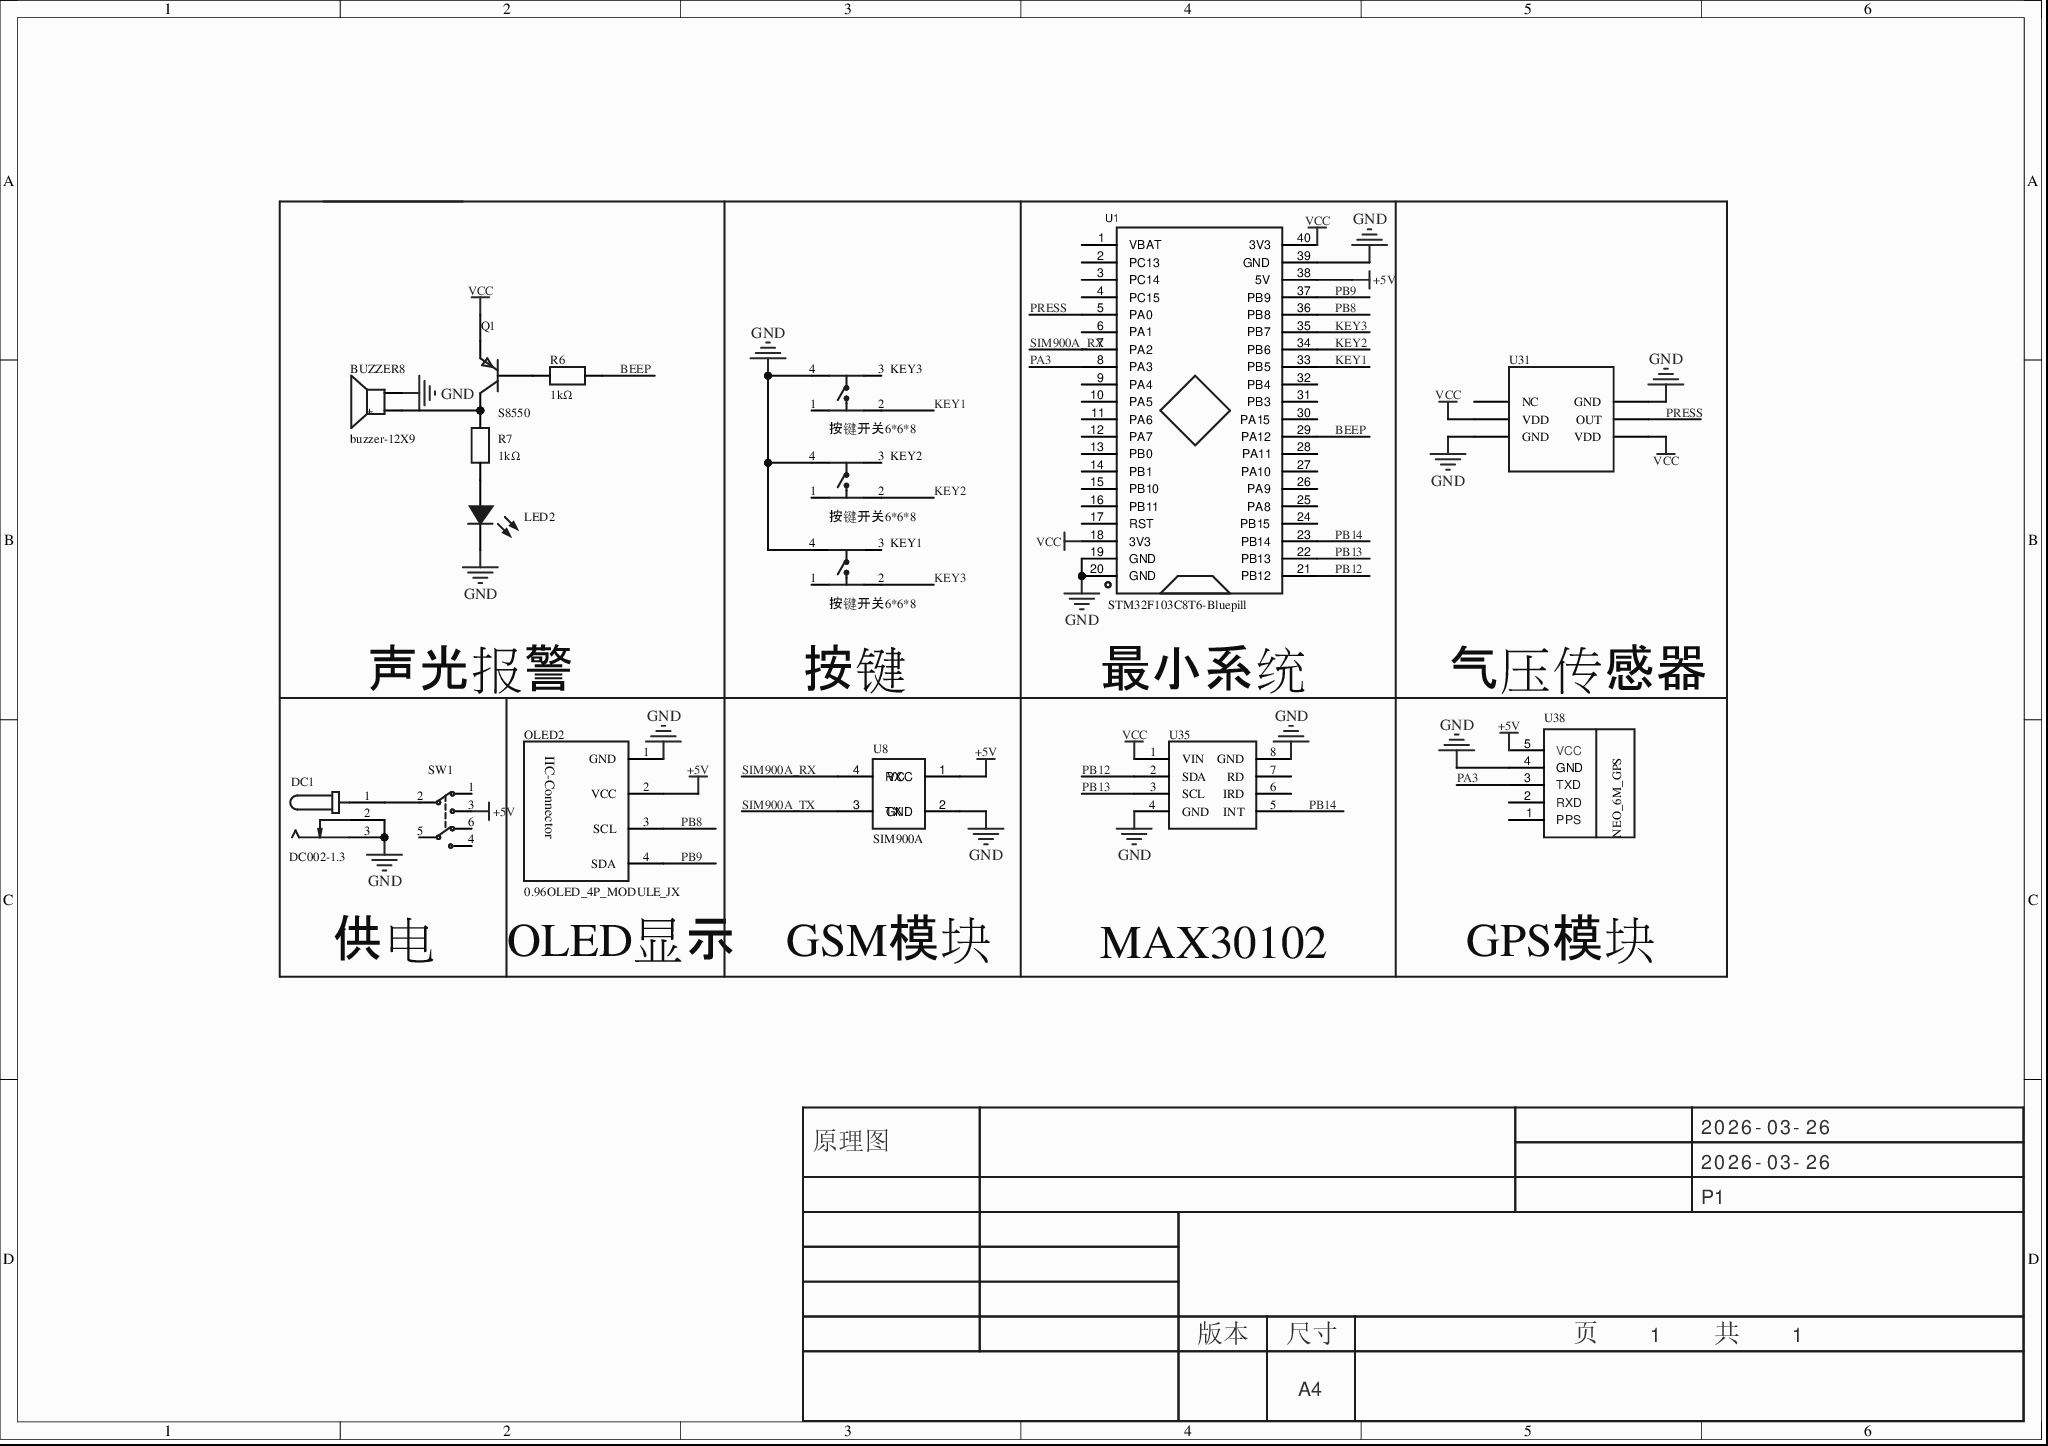
[diagram p0: MISC51078-3.schdoc]
# Altium project MISC51078-2.PrjPcb
1 sheet, 16 parts. Net scope: global (net labels, ports and power ports of the same name join across sheets).
Board file: MISC51078.pcbdoc

## Sheet MISC51078-3.schdoc
size 297 x 209 mm; Version: V1.0; @Project Name: MISC51078; @Page Count: 1; @Update Date: 2026-03-26; @Create Date: 2026-03-26; @Schematic Name: MISC51078; @Page No: 1; @Create Time: 13:47:48; @Update Time: 13:47:54; @Board Name: MISC51078

### Parts
BUZZER8  buzzer-12X9  [BUZ-TH_BD12.0-P7.60-D0.6-FD]
DC1  DC002-1.3  [DC-IN-TH_DC002-1.3]
KEY1  按键开关6*6*8  [KEY-TH_4P-L6.0-W6.0-P4.50-LS7.5]
KEY2  按键开关6*6*8  [KEY-TH_4P-L6.0-W6.0-P4.50-LS7.5]
KEY3  按键开关6*6*8  [KEY-TH_4P-L6.0-W6.0-P4.50-LS7.5]
LED2  (no value)  [LED_TH-3mm]
OLED2  0.96OLED_4P_MODULE_JX  [0.96OLED_4P]
Q1  S8550  [TO-92-3_L4.5-W3.5-P1.27-L]
R6  value 1kΩ  [RES-TH_BD2.3-L6.5-P10.50-D0.5]
R7  value 1kΩ  [RES-TH_BD2.3-L6.5-P10.50-D0.5]
SW1  (no value)  [自锁开关8.5*8.5]
U1  STM32F103C8T6-Bluepill  [STM32F103C8T6-BLUEPILL]
U8  SIM900A  [SIM900A]
U31  (no value)  [AGR12 表面压力传感器]
U35  (no value)  [MAX30102]
U38  (no value)  [NEO_6M_GPS模块]

### Nets
+5V: OLED2.2(VCC) SW1.3 U1.38(5V) U8.1(VCC) U38.5(VCC)
GND: BUZZER8.2 DC1.2 DC1.3 KEY1.4 KEY2.4 KEY3.4 LED2.2(A) OLED2.1(GND) U1.19(GND) U1.20(GND) U1.39(GND) U8.2(GND) U31.3(GND) U31.6(GND) U35.4(GND) U35.8(GND) U38.4(GND)
VCC: Q1.1(E) U1.18(3V3) U1.40(3V3) U31.2(VDD) U31.4(VDD) U35.1(VIN)
BEEP: R6.2 U1.29(PA12)
KEY1: KEY3.2 U1.33(PB5)
KEY2: KEY2.2 U1.34(PB6)
KEY3: KEY1.2 U1.35(PB7)
PA3: U1.8(PA3) U38.3(TXD)
PB8: OLED2.3(SCL) U1.36(PB8)
PB9: OLED2.4(SDA) U1.37(PB9)
PB12: U1.21(PB12) U35.2(SDA)
PB13: U1.22(PB13) U35.3(SCL)
PB14: U1.23(PB14) U35.5(INT)
PRESS: U1.5(PA0) U31.5(OUT)
SIM900A_RX: U1.7(PA2) U8.4(RX)
SIM900A_TX: U8.3(TX)
NetBUZZER8_1: BUZZER8.1(+) Q1.3(C) R7.2
NetDC1_1: DC1.1 SW1.2
NetLED2_1: LED2.1(C) R7.1
NetQ1_2: Q1.2(B) R6.1

Not connected (* = marked no-connect by the designer): KEY1 1 3; KEY2 1 3; KEY3 1 3; SW1 1* 4* 5* 6*; U1 1(VBAT) 2(PC13)* 3(PC14)* 4(PC15)* 6(PA1) 9(PA4) 10(PA5) 11(PA6) 12(PA7) 13(PB0) 14(PB1) 15(PB10) 16(PB11) 17(RST) 24(PB15) 25(PA8) 26(PA9) 27(PA10) 28(PA11) 30(PA15)* 31(PB3)* 32(PB4)*; U31 1(NC)*; U35 6(IRD)* 7(RD)*; U38 1(PPS)* 2(RXD)*

### Notes on the sheet
- 声光报警
- 按键
- 最小系统
- (near U38) 气压传感器
- 供电
- (near OLED2) OLED显示
- GSM模块
- MAX30102
- GPS模块
- 2026-03-26
- 原理图
- P1
- 版本
- 尺寸
- A4
- 页    1    共    1

### Library data of the parts
BUZZER8 = buzzer-12X9: AddInBom: yes; ModelId: 16ab50e14c5b4f2c986c135bdba60e37; ModelName: BUZ-TH_D12.0-H9.5-P7.60; ModelTransform: 472.4,472.2,0,90,0,0,-0.8,0,-177.2; Device: buzzer-12X9; Symbol: buzzer-12X9; LCSC Part Name: buzzer-12X9; SupplierPart: C9900016920; ManufacturerPart: buzzer-12X9; Supplier Footprint: BUZZER_SMT_9650B; JLCPCB Part Class: 扩展库; Datasheet: https://atta.szlcsc.comnull; Supplier: LCSC; ConvertToPcb: yes; FootprintName: BUZ-TH_BD12.0-P7.60-D0.6-FD
DC1 = DC002-1.3: Manufacturer: SHOU HAN(首韩); AddInBom: yes; ModelId: ccf1f99d79ab40ba9aeff26c21c7d5f1; ModelTransform: 208.661,472.44,0,0,0,0,-47.244,-100.748,-118.11; Device: DC002-1.3; Symbol: DC002-1.3; LCSC Part Name: DC座 DC-002 内芯1.3 圆针 3脚插件DC; SupplierPart: C668593; ManufacturerPart: DC002-1.3; Supplier Footprint: Through Hole; JLCPCB Part Class: 扩展库; Datasheet: https://atta.szlcsc.com/upload/public/pdf/source/20200619/C668593_6B5785499F122503841AA69BD23A954B.pdf; Supplier: LCSC; ConvertToPcb: yes; FootprintName: DC-IN-TH_DC002-1.3; ModelName: DC-IN-TH_DC002-1.3
KEY1-KEY3 = 按键开关6*6*8: 电路结构:SPST;触点额定电流:-;按钮头类型:Round Button;按钮作用方向:Top Actuated;; Symbol: button6*6*8; AddInBom: yes; ModelId: 84d39232fe0a426fa95ea2653754a6e5; ModelName: KEY-TH_4P-L6.0-W6.0-H4.5-LS6.5-P4.5; ModelTransform: 306.868,236.22,0,0,0,0,0,0,-118.11; Device: 按键开关6*6*8; LCSC Part Name: 按键开关6*6*8   直插; SupplierPart: C59982; ManufacturerPart: 按键开关6*6*8; Supplier Footprint: Through Hole; JLCPCB Part Class: 扩展库; Datasheet: https://atta.szlcsc.com/upload/public/pdf/source/20151126/1457707591845.pdf; Supplier: LCSC; ConvertToPcb: yes; FootprintName: KEY-TH_4P-L6.0-W6.0-P4.50-LS7.5
LED2 = LED_TH-B_3mm: ConvertToPcb: yes; ModelId: ff771fff7070432ca3f353cf0f67af4c0819f05c4eef4c71ace90d822a990e87; ModelName: LED-TH_BD3.8-P2.54-FD_BLUE; ModelTransform: 134.36,149.37,405.47,0,0,0,-11.81,0,-196.85; Device: LED_TH-B_3mm; Symbol: LED_TH-B; AddInBom: yes; Supplier Footprint: 插件; FootprintName: LED_TH-3mm
OLED2 = 0.96OLED_4P_MODULE_JX: AddInBom: yes; ModelId: 79c000fdb68d45a296c2e9bedf4f9055; ModelTransform: 1393.69792,1318.895,0,0,0,0,0,-560.079,-137.795; Device: 0.96OLED_4P_MODULE_JX; Symbol: 0.96OLED_4P_MODULE_JX; ConvertToPcb: yes; LCSC Part Name: 0.96OLED_4P_MODULE_JX; SupplierPart: C9900004566; ManufacturerPart: 0.96OLED_4P_MODULE_JX; Supplier Footprint: 插件; JLCPCB Part Class: 扩展库; Datasheet: https://atta.szlcsc.comnull; Supplier: LCSC; ModelName: 0.96OLED_4P; FootprintName: 0.96OLED_4P
Q1 = S8550_C2931493: Manufacturer: JSMSEMI(杰盛微); AddInBom: yes; ModelId: 45fa6cddef3743c6aacf8db740a3bc4c; ModelTransform: 177.165,137.795,0,0,0,0,0,29.528,-98.425; Device: S8550_C2931493; Symbol: S8550_C2931493; LCSC Part Name: S8550; SupplierPart: C2931493; ManufacturerPart: S8550; Supplier Footprint: TO-92; JLCPCB Part Class: 扩展库; Datasheet: https://atta.szlcsc.com/upload/public/pdf/source/20211216/FE7AA4A49EA39A06E5034A7E17568BAC.pdf; Supplier: LCSC; ConvertToPcb: yes; FootprintName: TO-92-3_L4.5-W3.5-P1.27-L; ModelName: TO-92-3_L4.5-W3.5-P1.27-L
R6 R7 = 插件电阻: 电阻类型:金属膜电阻;阻值:1kΩ;精度:±1%;功率:500mWS;温度系数:±50ppm/℃;工作温度范围:-;; Manufacturer: Tyohm(幸亚电阻); Symbol: RN1/2WS1KΩFT/BA1; AddInBom: yes; ModelId: 8e6c7ee8323443d1ab8f0504b6353c8c; ModelName: RES-TH_D2.3-L6.5-P10.50; ModelTransform: 431.1015,91.3384,0,0,0,0,0.197,0,-137.795; Tolerance: ±1%; Power(Watts): 500mWS; Device: 插件电阻; LCSC Part Name: 1kΩ ±1% 500mWS; SupplierPart: C385463; ManufacturerPart: RN1/2WS1KΩFT/BA1; Supplier Footprint: 轴向引线; JLCPCB Part Class: 扩展库; Datasheet: https://atta.szlcsc.com/upload/public/pdf/source/20190522/C385463_1A74B5322676C5D38AC622BB88C12821.pdf; Supplier: LCSC; ConvertToPcb: yes; FootprintName: RES-TH_BD2.3-L6.5-P10.50-D0.5; Type: 金属膜电阻; Temperature Coefficient: ±50ppm/℃; Operating Temperature Range: -
SW1 = 自锁开关: ConvertToPcb: yes; ModelId: afccd99c58414b25b20cb6a0f4e08c2e; ModelName: self_switch; ModelTransform: 287.4,287.4,673.9,0,0,0,90.55,-100,-161.42; Device: 自锁开关; Symbol: 自锁开关; AddInBom: yes; FootprintName: 自锁开关8.5*8.5
U1 = STM32F103C8T6-Bluepill: AddInBom: yes; Symbol: STM32F103C8T6-Bluepill; Device: STM32F103C8T6-Bluepill; FootprintName: STM32F103C8T6-BLUEPILL; ConvertToPcb: yes
U8 = SIM900A: AddInBom: yes; _: 3; Device: SIM900A; Symbol: SIM900A; ConvertToPcb: yes; FootprintName: SIM900A
U31 = AGR12 表面压力传感器: AddInBom: yes; Device: AGR12 表面压力传感器; Symbol: AGR12 表面压力传感器; ConvertToPcb: yes; FootprintName: AGR12 表面压力传感器
U35 = MAX30102: AddInBom: yes; Pin Type: IN; ModelId: be9d53a4952f410699548e9c532bf609; ModelName: MAX30102模块; ModelTransform: 614.17,807.08,98.43,0,0,0,0,0,0; _: 3; Symbol: MAX30102; Device: MAX30102; ConvertToPcb: yes; FootprintName: MAX30102
U38 = NEO_6M_GPS模块: GPS定位模块，串口通信; Add into BOM: yes; Device: NEO_6M_GPS模块; Convert to PCB: yes; Symbol: NEO_6M_GPS模块; FootprintName: NEO_6M_GPS模块; JLCPCB Part Class: 扩展库